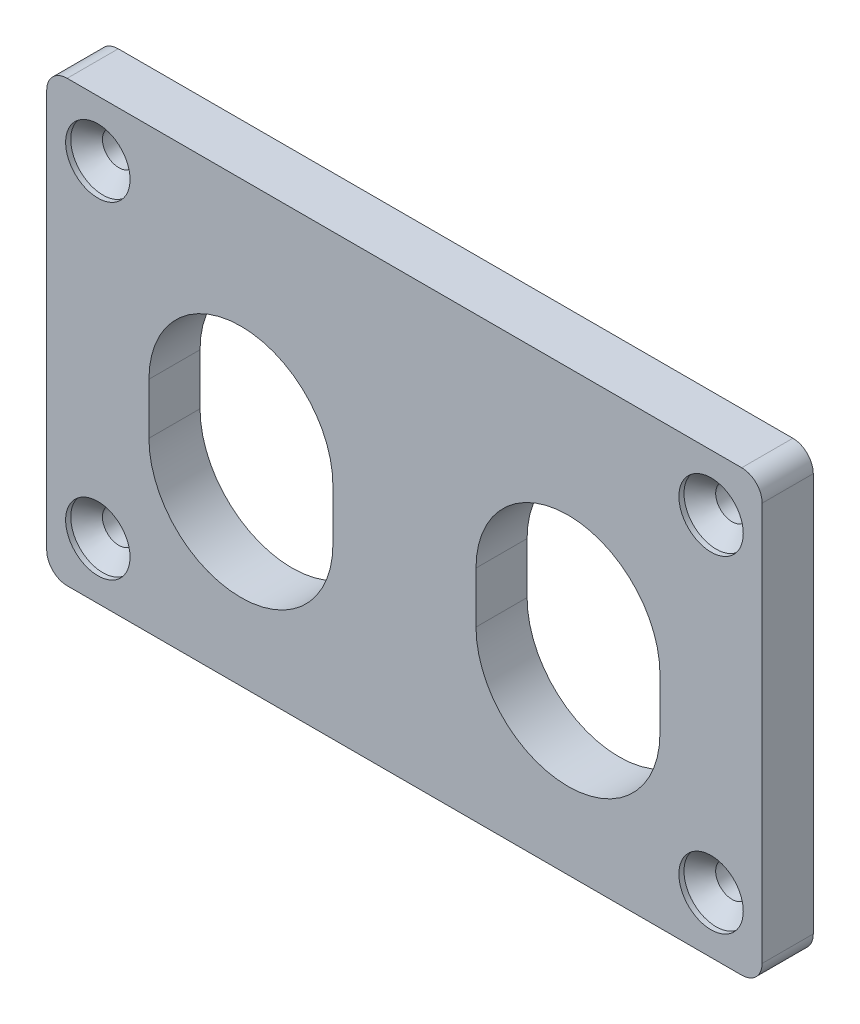
from build123d import *

# Parameters (mm, degrees)
BOSS_EXTRUDE1_DEPTH                            = 5
CSK_FOR_M3_FLAT_HEAD_MACHINE_SCREW1_AT_2_COUNT = 2
CSK_FOR_M3_FLAT_HEAD_MACHINE_SCREW1_AT_2_PITCH = 32
CSK_FOR_M3_FLAT_HEAD_MACHINE_SCREW1_AT_3_COUNT = 2
CSK_FOR_M3_FLAT_HEAD_MACHINE_SCREW1_AT_3_PITCH = 68
CSK_FOR_M3_FLAT_HEAD_MACHINE_SCREW1_AT_4_COUNT = 2
CSK_FOR_M3_FLAT_HEAD_MACHINE_SCREW1_AT_4_PITCH = 60


with BuildPart() as part:
    # Sketch1 → Boss-Extrude1 (new body)
    with BuildSketch(Plane.XY):
        with BuildLine():
            Line((2, 0), (68, 0))
            ThreePointArc((68, 0), (69.414213562, 0.585786438), (70, 2))
            Line((70, 2), (70, 41))
            ThreePointArc((70, 41), (69.414213562, 42.414213562), (68, 43))
            Line((68, 43), (2, 43))
            ThreePointArc((2, 43), (0.585786438, 42.414213562), (0, 41))
            Line((0, 41), (0, 2))
            ThreePointArc((0, 2), (0.585786438, 0.585786438), (2, 0))
        make_face()
        with BuildLine():
            Line((28, 21.5), (28, 16.5))
            ThreePointArc((28, 16.5), (19, 7.5), (10, 16.5))
            Line((10, 16.5), (10, 21.5))
            ThreePointArc((10, 21.5), (19, 30.5), (28, 21.5))
        make_face(mode=Mode.SUBTRACT)
        with BuildLine():
            Line((60, 21.5), (60, 16.5))
            ThreePointArc((60, 16.5), (51, 7.5), (42, 16.5))
            Line((42, 16.5), (42, 21.5))
            ThreePointArc((42, 21.5), (51, 30.5), (60, 21.5))
        make_face(mode=Mode.SUBTRACT)
    extrude(amount=BOSS_EXTRUDE1_DEPTH)

    # Sketch2 → CSK for M3 Flat Head Machine Screw1 (revolve, cut)
    with BuildSketch(Plane(origin=(5, 37.5, 5), x_dir=(0, -1, 0), z_dir=(1, 0, 0))):
        Polygon((0, 0), (0, 5), (1.6, 5), (1.6, 2.05), (3.15, 0.5), (3.15, 0), align=None)
    csk_for_m3_flat_head_machine_screw1 = revolve(axis=Axis((5, 37.5, 11.35), (0, 0, -1)), mode=Mode.SUBTRACT)

    # CSK for M3 Flat Head Machine Screw1 at 2: CSK for M3 Flat Head Machine Screw1 ×2
    with Locations(*[(0, -i * CSK_FOR_M3_FLAT_HEAD_MACHINE_SCREW1_AT_2_PITCH, 0) for i in range(1, CSK_FOR_M3_FLAT_HEAD_MACHINE_SCREW1_AT_2_COUNT)]):
        add(csk_for_m3_flat_head_machine_screw1, mode=Mode.SUBTRACT)

    # CSK for M3 Flat Head Machine Screw1 at 3: CSK for M3 Flat Head Machine Screw1 ×2
    with Locations(*[Vector(0.8823529411764707, -0.47058823529411764, 0) * (i * CSK_FOR_M3_FLAT_HEAD_MACHINE_SCREW1_AT_3_PITCH) for i in range(1, CSK_FOR_M3_FLAT_HEAD_MACHINE_SCREW1_AT_3_COUNT)]):
        add(csk_for_m3_flat_head_machine_screw1, mode=Mode.SUBTRACT)

    # CSK for M3 Flat Head Machine Screw1 at 4: CSK for M3 Flat Head Machine Screw1 ×2
    with Locations(*[(i * CSK_FOR_M3_FLAT_HEAD_MACHINE_SCREW1_AT_4_PITCH, 0, 0) for i in range(1, CSK_FOR_M3_FLAT_HEAD_MACHINE_SCREW1_AT_4_COUNT)]):
        add(csk_for_m3_flat_head_machine_screw1, mode=Mode.SUBTRACT)


solid = part.part
